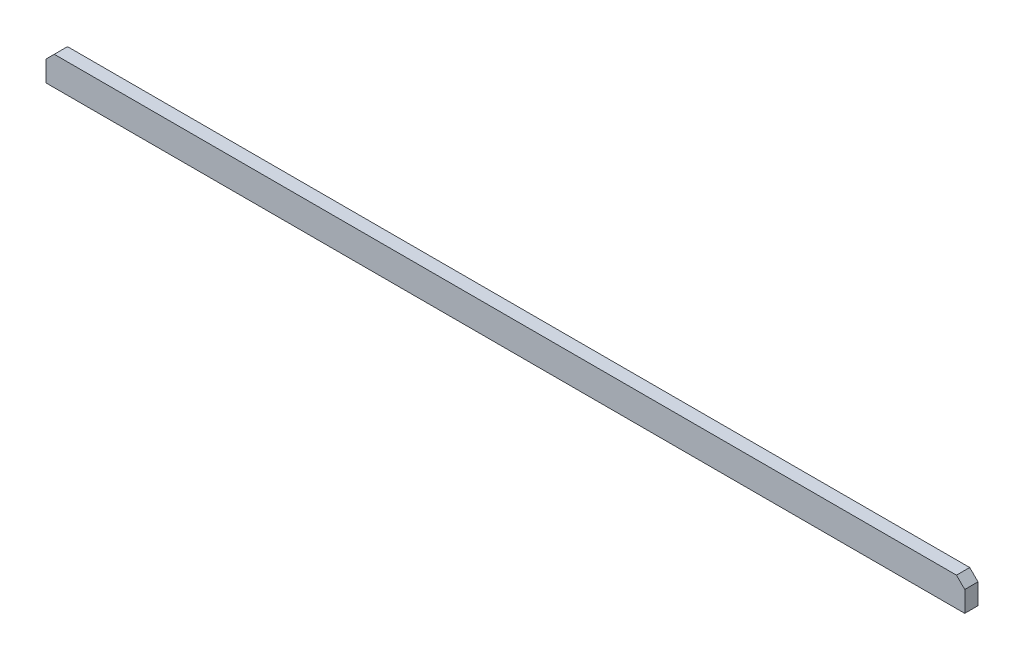
SolidWorks part; units mm, degrees
ref_plane "Front Plane" through (0, 0, 0) normal (0, 0, 1) x (1, 0, 0)
ref_plane "Top Plane" through (0, 0, 0) normal (0, 1, 0) x (1, 0, 0)
ref_plane "Right Plane" through (0, 0, 0) normal (1, 0, 0) x (0, 0, -1)
sketch "Sketch1" plane through (0, 0, 0) normal (0, 0, 1) x (1, 0, 0)
  line L0 (-64.5136, 32.6234) -> (-64.5136, -2.3766)
  line L1 (-64.5136, -2.3766) -> (1045.4864, -2.3766)
  line L2 (1045.4864, -2.3766) -> (1045.4864, 32.6234)
  line L3 (1045.4864, 32.6234) -> (-64.5136, 32.6234)
extrude "Boss-Extrude1" add sketch "Sketch1" along normal blind 16
chamfer "Chamfer1" distance 10 angle 45 2 edges at (1045.4864, 32.6234, 8) (-64.5136, 32.6234, 8)
